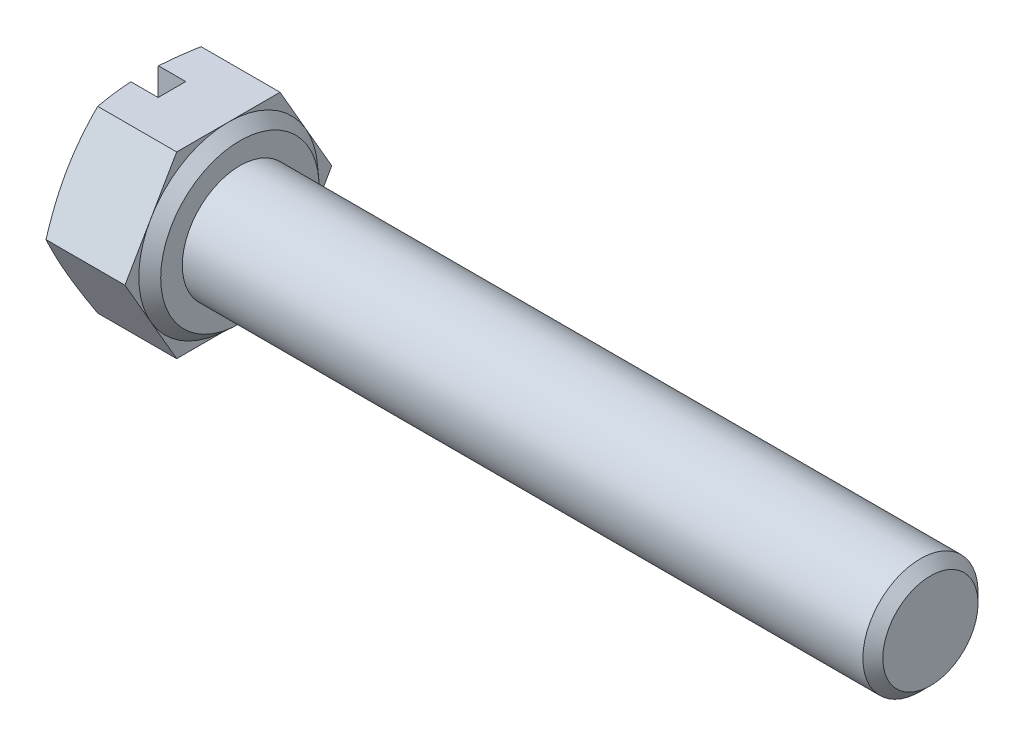
SolidWorks part; units mm, degrees
ref_plane "Front" through (0, 0, 0) normal (0, 0, 1) x (1, 0, 0)
ref_plane "Top" through (0, 0, 0) normal (0, 1, 0) x (1, 0, 0)
ref_plane "Right" through (0, 0, 0) normal (1, 0, 0) x (0, 0, -1)
other "Configuration Table"
sketch "Sketch-BaseHead" plane through (0, 0, 0) normal (1, 0, 0) x (0, 0, -1)
  line L1 (2.2459, -3.89) -> (4.4918, 0)
  line L2 (4.4918, 0) -> (2.2459, 3.89)
  line L3 (2.2459, 3.89) -> (-2.2459, 3.89)
  line L4 (-2.2459, 3.89) -> (-4.4918, 0)
  line L5 (-4.4918, 0) -> (-2.2459, -3.89)
  line L6 (-2.2459, -3.89) -> (2.2459, -3.89)
  circle A0 centre (0, 0) radius 3.89 construction
extrude "BaseHead" add sketch "Sketch-BaseHead" along normal blind 3.65
ref_plane "Plane1" through (4.15, 0, 0) normal (1, 0, 0) x (0, 0, -1)
sketch "Sketch1" plane through (0, 0, 0) normal (0, 0, 1) x (1, 0, 0)
  line L0 (3.65, 0) -> (4.15, 0)
  line L1 (4.15, 0) -> (4.15, -3.44)
  line L2 (4.15, -3.44) -> (3.65, -3.89)
  line L3 (3.65, -3.89) -> (3.65, 0)
revolve "Revolve1" add sketch "Sketch1" angle 360 about axis through (-4.0016, 0, 0) along (1, 0, 0)
sketch "Sketch3" plane through (4.15, 0, 0) normal (1, 0, 0) x (0, 0, -1)
  circle A0 centre (0, 0) radius 2.5
extrude "BaseBody" add sketch "Sketch3" along normal blind 30
cosmetic thread "ThreadCosmetic1" parameters "D2"=4.134
chamfer "Chamfer1" distance 0.433 angle 45 1 edges at (34.15, 0, -2.5)
fillet "HeadFillet" [suppressed] radius 0.2
sketch "Sketch4" plane through (-0.2646, 0, 5.9169) normal (0, 1, 0) x (0, 0, -1)
  line L0 (5.9169, 3.7369) -> (5.9169, -10.4477) construction
  line L2 (10.4087, -0.2646) -> (9.8069, -0.2646)
  line L4 (9.8069, -0.2646) -> (10.4087, -0.4837)
  line L6 (10.4087, -0.4837) -> (10.4087, -0.2646)
revolve "HeadChamfer" cut sketch "Sketch4" angle 360 about L0
sketch "Sketch5" plane through (0, 0, 0) normal (0, 1, 0) x (1, 0, 0)
  line L0 (0, 0.6) -> (0, -0.6)
  line L1 (1.2, -0.6) -> (1.2, 0.6)
  line L2 (1.2, 0.6) -> (0, 0.6)
  line L3 (0, -0.6) -> (1.2, -0.6)
  dimension "n" = 1.2
  dimension "t" = 1.2
extrude "Slot" cut sketch "Sketch5" against normal through all and the other way through all
sketch "Sketch6" plane through (0, 0, 0) normal (0, 0, 1) x (1, 0, 0)
  line L0 (4.15, 2.7) -> (4.583, 2.7)
  line L1 (4.583, 2.7) -> (4.583, 2.5)
  line L2 (4.583, 2.5) -> (4.3665, 2.125)
  line L3 (4.15, 2.5) -> (4.3665, 2.125)
  line L4 (4.15, 2.7) -> (4.15, 2.5)
  line L5 (14.0487, 0) -> (0, 0) construction
  line L6 (4.15, 2.5) -> (4.583, 2.5) construction
  line L7 (4.3665, 2.5) -> (4.3665, 2.125) construction
  point P5 (4.3665, 2.7)
revolve "Cut-Revolve10" [suppressed] cut sketch "Sketch6" angle 360 about L5
pattern_linear "LPattern10" [suppressed] count 58 spacing 0.5196
equation "\"D1@Sketch1\" = \"s@Sketch-BaseHead\"/ 2 "
equation "\"D2@Sketch4\" = \"s@Sketch-BaseHead\""
equation "\"D1@Chamfer1\" =  ( \"d@Sketch3\" - \"D2@ThreadCosmetic1\" ) / 2 "
equation "\"D2@Sketch6\" = (  \"d@Sketch3\" - \"D2@ThreadCosmetic1\" )  / 2"
equation "\"D3@LPattern10\" = \"D2@Sketch6\" * 1.2"
equation "\"D1@LPattern10\" = \"l@BaseBody\" / \"D3@LPattern10\""
